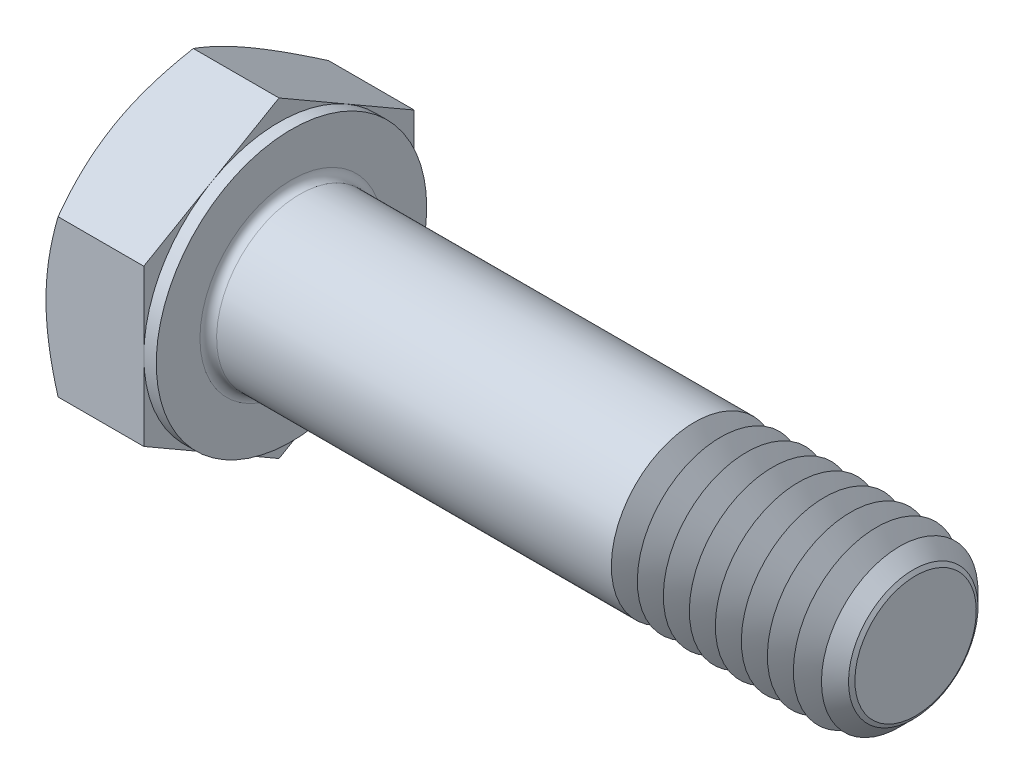
from build123d import *

# Parameters (mm, degrees)
EXTRUDE_378_DEPTH      = 5.3
SKETCH_4_W             = 0.6
SKETCH_4_H             = 11.005553499
CHAMFER_2060_SIZE      = 1
FILLET_2105_R          = 0.4
PATTERN_LINEAR_1_COUNT = 9
PATTERN_LINEAR_1_PITCH = 1.25


with BuildPart() as part:
    # 草图1 → Extrude 378 (new body)
    with BuildSketch(Plane(origin=(0, 0, 0), x_dir=(0, 0, -1), z_dir=(1, 0, 0))):
        Polygon((6.5, 3.75277675), (6.5, -3.75277675), (0, -7.505553499), (-6.5, -3.75277675), (-6.5, 3.75277675), (0, 7.505553499), align=None)
    extrude(amount=EXTRUDE_378_DEPTH)

    # 草图2 → 凸台-旋转1 (revolve)
    with BuildSketch(Plane.XY, mode=Mode.PRIVATE) as revolve_1_sk:
        Polygon((0, 0), (35.3, 0), (35.3, 2.9175), (35.3, 4), (7.791693541, 4), (0, 4), align=None)
    revolve(revolve_1_sk.sketch.rotate(Axis((0, 0, 0), (1, 0, 0)), 90), axis=Axis((0, 0, 0), (1, 0, 0)))

    # 草图3 → 切除-旋转1 (revolve, cut)
    with BuildSketch(Plane.XY):
        Polygon((0, 6.5), (3.46730793, 12.505553499), (3.46730793, 17.505553499), (-10, 17.505553499), (-10, 6.5), align=None)
    revolve(axis=Axis((0, 0, 0), (1, 0, 0)), mode=Mode.SUBTRACT)

    # 草图5 → 切除-旋转2 (revolve, cut)
    with BuildSketch(Plane.XY):
        Polygon((5.3, 6.5), (1.83269207, 12.505553499), (1.83269207, 17.505553499), (11.83269207, 17.505553499), (11.83269207, 6.5), align=None)
    revolve(axis=Axis((0, 0, 0), (1, 0, 0)), mode=Mode.SUBTRACT)

    # 草图4 → 切除-旋转3 (revolve, cut)
    with BuildSketch(Plane.XY, mode=Mode.PRIVATE) as cut_revolve_3_sk:
        with Locations((5, 12.00277675)):
            Rectangle(SKETCH_4_W, SKETCH_4_H)
    revolve(cut_revolve_3_sk.sketch.rotate(Axis((0, 0, 0), (1, 0, 0)), 270), axis=Axis((0, 0, 0), (1, 0, 0)), mode=Mode.SUBTRACT)

    # Chamfer 2060
    chamfer_2060_edges = [part.edges().sort_by_distance(p)[0] for p in [
        (35.3, 0, -4),
    ]]
    chamfer(chamfer_2060_edges, length=CHAMFER_2060_SIZE)

    # Fillet 2105
    fillet_2105_edges = [part.edges().sort_by_distance(p)[0] for p in [
        (5.3, 0, -4),
    ]]
    fillet(fillet_2105_edges, radius=FILLET_2105_R)

    # 草图6 → 切除-旋转4 (revolve, cut)
    with BuildSketch(Plane.XY):
        Polygon((25.3, -2.9175), (24.675018334, -4), (24.675018334, -5), (25.924981666, -5), (25.924981666, -4), align=None)
    cut_revolve_4 = revolve(axis=Axis((-3.175, 0, 0), (1, 0, 0)), mode=Mode.SUBTRACT)

    # 阵列(线性)1: 切除-旋转4 ×9
    with Locations(*[(i * PATTERN_LINEAR_1_PITCH, 0, 0) for i in range(1, PATTERN_LINEAR_1_COUNT)]):
        add(cut_revolve_4, mode=Mode.SUBTRACT)


solid = part.part
